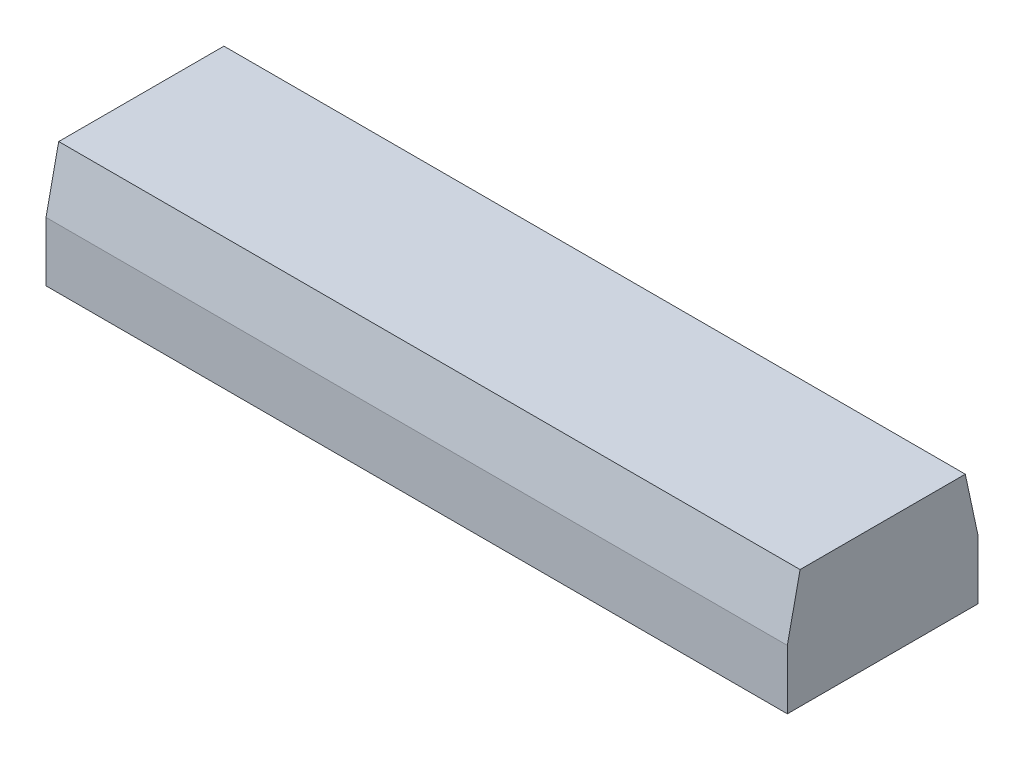
from build123d import *

# Parameters (mm, degrees)
SKETCH1_W             = 175
SKETCH1_H             = 28
BOSS_EXTRUDE1_DEPTH   = 45
M8_TAPPED_HOLE1_D     = 6.8
M8_TAPPED_HOLE1_DEPTH = 19.75
M8_TAPPED_HOLE1_TIP   = 2.042926105
CUT_EXTRUDE1_DEPTH    = 183.849665026


with BuildPart() as part:
    # Sketch1 → Boss-Extrude1 (new body)
    with BuildSketch(Plane.XY):
        with Locations((87.5, -14)):
            Rectangle(SKETCH1_W, SKETCH1_H)
    extrude(amount=BOSS_EXTRUDE1_DEPTH)

    # M8 Tapped Hole1
    with Locations(Plane(origin=(0, -28, 0), x_dir=(-1, 0, 0), z_dir=(0, -1, 0))):
        with Locations((-27.5, -21), (-147.5, -21)):
            Hole(M8_TAPPED_HOLE1_D / 2, depth=M8_TAPPED_HOLE1_DEPTH)
            with Locations((0, 0, -(M8_TAPPED_HOLE1_DEPTH + M8_TAPPED_HOLE1_TIP / 2))):  # 118° drill point
                Cone(0, M8_TAPPED_HOLE1_D / 2, M8_TAPPED_HOLE1_TIP, mode=Mode.SUBTRACT)

    # Sketch7 → Cut-Extrude1 (cut, through all)
    with BuildSketch(Plane.ZY):
        Polygon((3, 0), (0, -14), (0, 0), align=None)
        Polygon((45, 0), (42, 0), (45, -14), align=None)
    extrude(amount=-CUT_EXTRUDE1_DEPTH, mode=Mode.SUBTRACT)


solid = part.part
